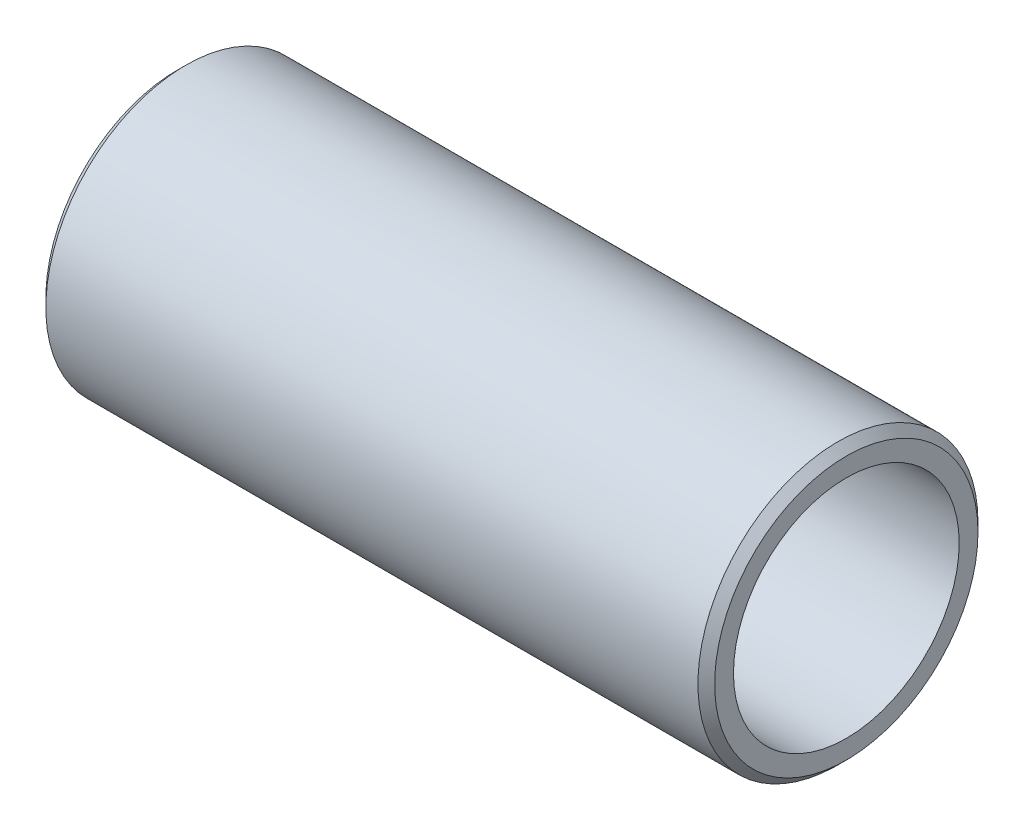
from build123d import *

# Parameters (mm, degrees)
SKETCH_1_R      = 16.75
SKETCH_1_R_2    = 13.5
EXTRUDE_1_DEPTH = 80
CHAMFER_1_SIZE  = 1


with BuildPart() as part:
    # 草图1 → 拉伸-薄壁1 (new body)
    with BuildSketch(Plane(origin=(0, 0, 0), x_dir=(0, 0, -1), z_dir=(1, 0, 0))):
        Circle(SKETCH_1_R)
        Circle(SKETCH_1_R_2, mode=Mode.SUBTRACT)
    extrude(amount=EXTRUDE_1_DEPTH)

    # 倒角1
    chamfer_1_edges = [part.edges().sort_by_distance(p)[0] for p in [
        (0, 0, 16.75),
        (80, 0, 16.75),
    ]]
    chamfer(chamfer_1_edges, length=CHAMFER_1_SIZE)


solid = part.part
